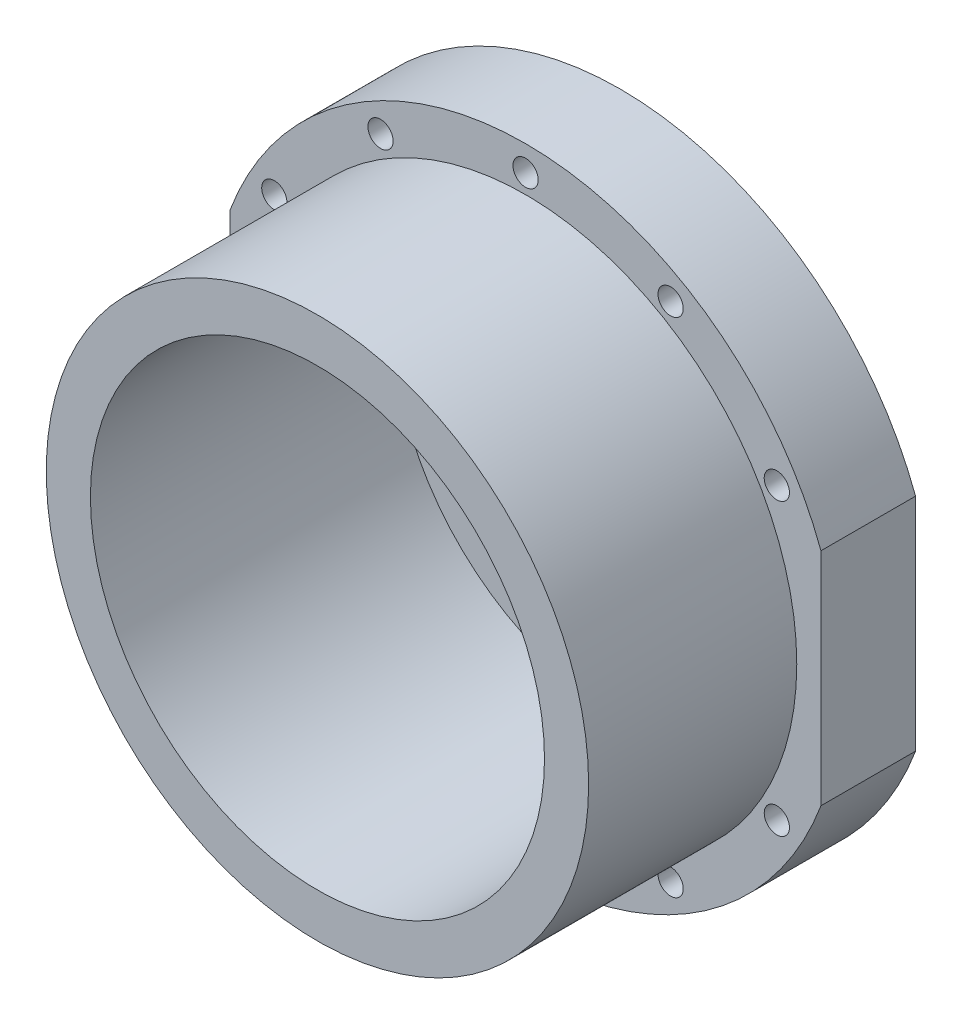
SolidWorks part; units mm, degrees
ref_plane "Front Plane" through (0, 0, 0) normal (0, 0, 1) x (1, 0, 0)
ref_plane "Top Plane" through (0, 0, 0) normal (0, 1, 0) x (1, 0, 0)
ref_plane "Right Plane" through (0, 0, 0) normal (1, 0, 0) x (0, 0, -1)
other "Configuration Table"
sketch "Sketch1" plane through (0, 0, 0) normal (0, 0, 1) x (1, 0, 0)
  circle A0 centre (0, 0) radius 36
  circle A1 centre (0, 0) radius 50
  dimension "D1" = 72
  dimension "D2" = 100
extrude "Boss-Extrude1" add sketch "Sketch1" along normal blind 15
sketch "Sketch2" plane through (0, 0, 15) normal (0, 0, 1) x (1, 0, 0)
  line L0 (0, -58.9645) -> (0, 58.9645) construction
  line L1 (-46.835, 17.5066) -> (-46.835, -17.5066)
  line L2 (46.835, 17.5066) -> (46.835, -17.5066)
  circle A0 centre (0, 0) radius 50 construction
  arc A1 (-46.835, 17.5066) -> (-46.835, -17.5066) centre (0, 0) ccw
  arc A2 (46.835, -17.5066) -> (46.835, 17.5066) centre (0, 0) ccw
  point P6 (0, 0)
  dimension "D1" = 93.67
extrude "Cut-Extrude1" cut sketch "Sketch2" against normal blind 48
sketch "Sketch4" plane through (0, 0, 0) normal (0, 0, -1) x (-1, 0, 0)
  circle A0 centre (0, 0) radius 30
  circle A1 centre (0, 0) radius 40
  dimension "D1" = 60
  dimension "D2" = 80
extrude "Boss-Extrude2" add sketch "Sketch4" along normal blind 5
sketch "Sketch5" plane through (0, 0, 15) normal (0, 0, 1) x (1, 0, 0)
  circle A0 centre (0, 0) radius 36
  circle A1 centre (0, 0) radius 43
  dimension "D1" = 72
  dimension "D2" = 86
extrude "Boss-Extrude3" add sketch "Sketch5" along normal blind 33
sketch "Sketch6" plane through (0, 0, 15) normal (0, 0, 1) x (1, 0, 0)
  line L0 (-68.7099, 0) -> (68.7099, 0) construction
  circle A0 centre (0, 46) radius 2
  circle A1 centre (39.8372, -23) radius 2
  circle A2 centre (23, 39.8372) radius 2
  circle A3 centre (39.8372, 23) radius 2
  circle A4 centre (-23, 39.8372) radius 2
  circle A5 centre (-39.8372, 23) radius 2
  circle A6 centre (23, -39.8372) radius 2
  circle A7 centre (0, -46) radius 2
  circle A8 centre (-23, -39.8372) radius 2
  circle A9 centre (-39.8372, -23) radius 2
  point P9 (0, 0)
  point P14 (0, 0)
  point P16 (0, 0)
  dimension "D1" = 4
  dimension "D2" = 46
  dimension "D3" = 3
  dimension "D4" = 3
extrude "Cut-Extrude2" cut sketch "Sketch6" against normal blind 30
